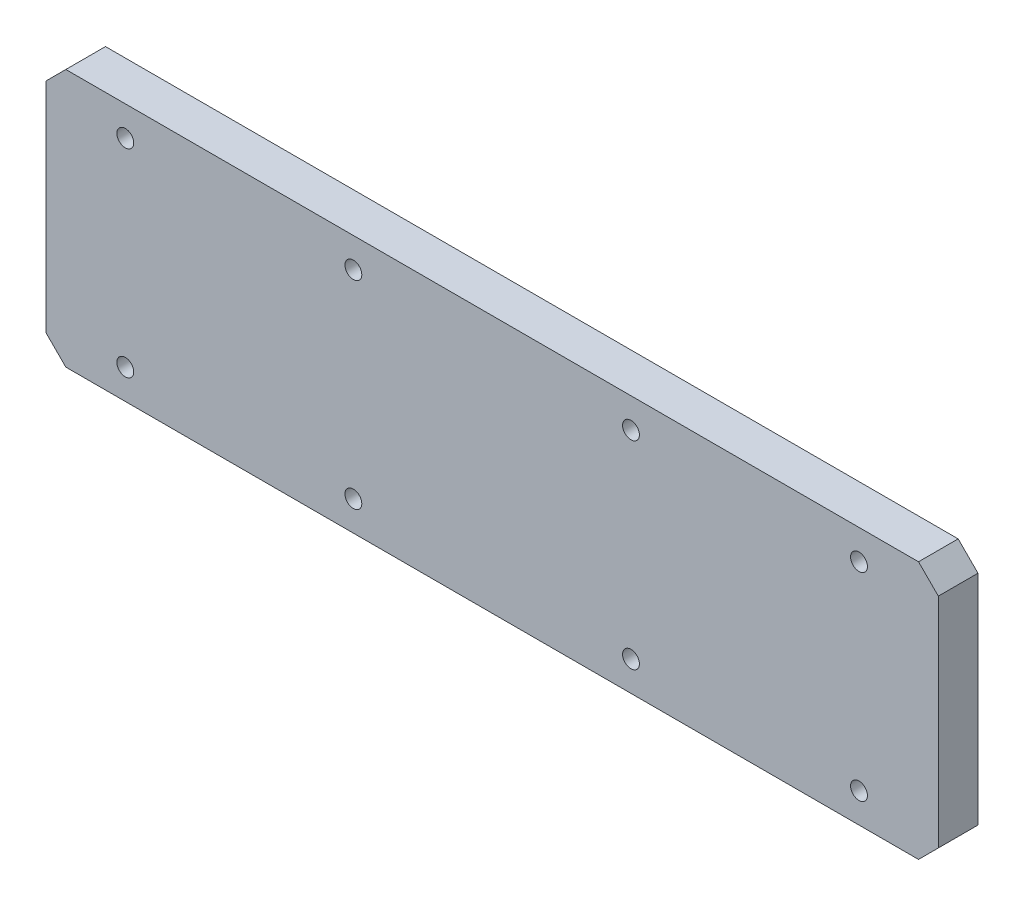
SolidWorks part; units mm, degrees
material "Q235A"
ref_plane "Front Plane" through (0, 0, 0) normal (0, 0, 1) x (1, 0, 0)
ref_plane "Top Plane" through (0, 0, 0) normal (0, 1, 0) x (1, 0, 0)
ref_plane "Right Plane" through (0, 0, 0) normal (1, 0, 0) x (0, 0, -1)
sketch "Sketch1" plane through (0, 0, 0) normal (0, 0, 1) x (1, 0, 0)
  line L1 (450, -130) -> (-450, -130)
  line L2 (450, -130) -> (450, 130)
  line L3 (450, 130) -> (-450, 130)
  line L4 (-450, -130) -> (-450, 130)
  line L5 (450, -130) -> (-450, 130) construction
  line L6 (450, 130) -> (-450, -130) construction
  point P0 (0, 0)
  dimension "D1" = 900
  dimension "D2" = 260
extrude "Boss-Extrude1" add sketch "Sketch1" along normal blind 40
hole_wizard "Ø17.0 (17) Diameter Hole1" positions "Sketch2" profile "Sketch3" hole size "Ø17.0" standard "GB"
sketch "Sketch2" plane through (0, 0, 40) normal (0, 0, 1) x (1, 0, 0)
  line L0 (0, 130) -> (0, 0) construction
  line L1 (450, 130) -> (-450, 130) construction
  line L2 (0, 0) -> (-459.0951, 0) construction
  line L4 (-450, 130) -> (-450, -130) construction
  point P0 (-370, 100)
  point P2 (-140, 100)
  point P14 (-370, -100)
  point P15 (-140, -100)
  point P16 (140, -100)
  point P17 (370, -100)
  point P18 (140, 100)
  point P19 (370, 100)
  dimension "D1" = 80
  dimension "D2" = 280
  dimension "D3" = 200
sketch "Sketch3" plane through (-370, 100, 40) normal (1, 0, 0) x (0, -1, 0)
  line L0 (0, 0) -> (0, 47.1073)
  line L1 (0, 47.1073) -> (8.5, 42)
  line L2 (8.5, 42) -> (8.5, 0)
  line L5 (8.5, 0) -> (0, 0)
  line L10 (0, 47.1073) -> (-8.5, 42) construction
  line L11 (0, -6.35) -> (0, 107.95) construction
  dimension "孔直径" = 17
  dimension "孔深度" = 42
  dimension "导头角度" = 118
chamfer "Chamfer1" distance 20 angle 45 4 edges at (-450, 130, 20) (450, 130, 20) (450, -130, 20) (-450, -130, 20)
